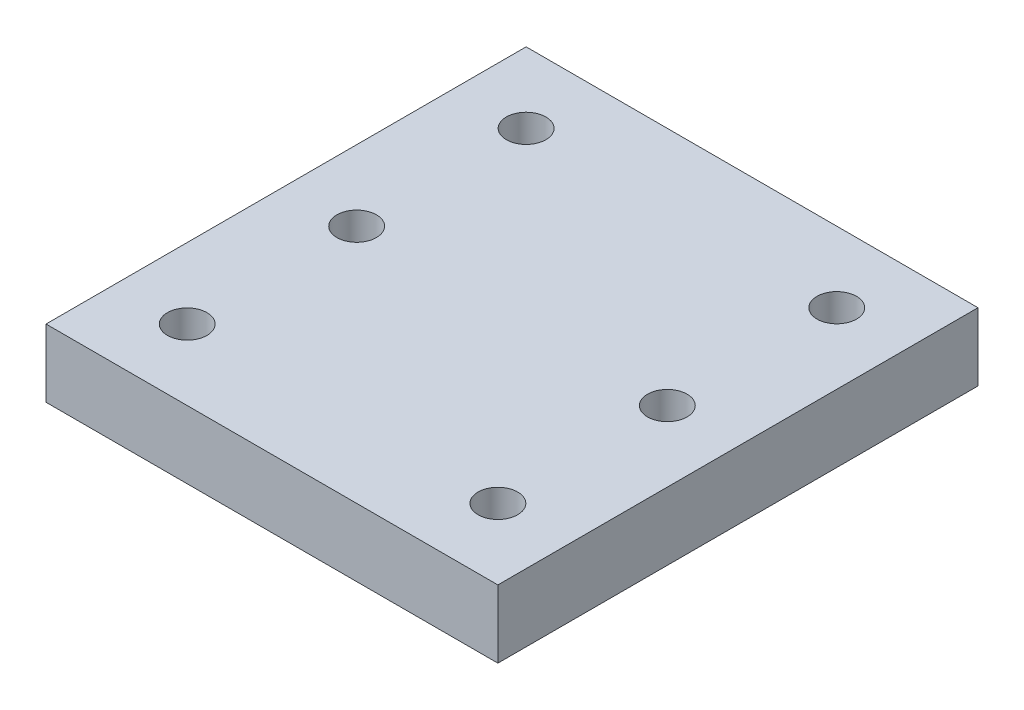
SolidWorks part; units mm, degrees
material "A3"
ref_plane "前视基准面" through (0, 0, 0) normal (0, 0, 1) x (1, 0, 0)
ref_plane "上视基准面" through (0, 0, 0) normal (0, 1, 0) x (1, 0, 0)
ref_plane "右视基准面" through (0, 0, 0) normal (1, 0, 0) x (0, 0, -1)
sketch "草图1" plane through (0, 0, 0) normal (0, 1, 0) x (1, 0, 0)
  line L1 (-80, -85) -> (80, -85)
  line L2 (-80, -85) -> (-80, 85)
  line L3 (-80, 85) -> (80, 85)
  line L4 (80, -85) -> (80, 85)
  line L5 (-80, -85) -> (80, 85) construction
  line L6 (-80, 85) -> (80, -85) construction
  point P0 (0, 0)
  dimension "D1" = 170
  dimension "D2" = 160
extrude "凸台-拉伸1" add sketch "草图1" along normal blind 24
hole_wizard "M16 螺纹孔1" positions "草图2" profile "草图3" tap size "M16" standard "GB" end condition through all
sketch "草图2" plane through (0, 24, 0) normal (0, 1, 0) x (1, 0, 0)
  line L0 (0, 85) -> (0, 0) construction
  line L1 (80, 85) -> (-80, 85) construction
  line L2 (0, 0) -> (80, 0) construction
  line L3 (80, -85) -> (80, 85) construction
  point P0 (-55, -60)
  point P14 (-55, 60)
  point P15 (55, 60)
  point P16 (55, -60)
  point P17 (55, 0)
  point P21 (-55, 0)
  dimension "D1" = 110
  dimension "D2" = 120
sketch "草图3" plane through (-55, 24, 60) normal (1, 0, 0) x (0, 0, 1)
  line L0 (0, 0) -> (0, 24)
  line L1 (0, 24) -> (7, 24)
  line L2 (7, 24) -> (7, 0)
  line L5 (7, 0) -> (0, 0)
  line L11 (0, -6.35) -> (0, 107.95) construction
  dimension "通孔螺纹孔钻头直径" = 14
  dimension "通孔螺纹孔钻头深度" = 24
cosmetic thread "孔螺蚊线1" parameters "D2"=16
cosmetic thread "孔螺蚊线2" parameters "D2"=16
cosmetic thread "孔螺蚊线3" parameters "D2"=16
cosmetic thread "孔螺蚊线4" parameters "D2"=16
cosmetic thread "孔螺蚊线5" parameters "D2"=16
cosmetic thread "孔螺蚊线6" parameters "D2"=16
